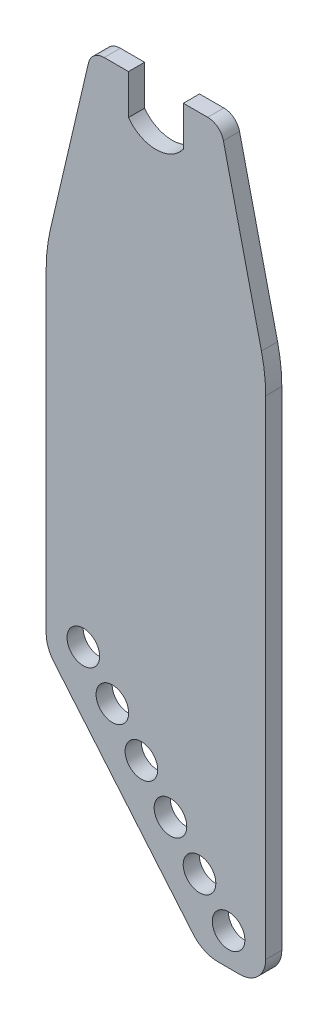
SolidWorks part; units mm, degrees
material "45#"
ref_plane "Front Plane" through (0, 0, 0) normal (0, 0, 1) x (1, 0, 0)
ref_plane "Top Plane" through (0, 0, 0) normal (0, 1, 0) x (1, 0, 0)
ref_plane "Right Plane" through (0, 0, 0) normal (1, 0, 0) x (0, 0, -1)
sketch "Sketch1" plane through (0, 0, 0) normal (0, 0, 1) x (1, 0, 0)
  line L1 (-34, 112.5) -> (34, 112.5)
  line L2 (-34, 112.5) -> (-34, -112.5)
  line L3 (-34, -112.5) -> (34, -112.5)
  line L4 (34, 112.5) -> (34, -112.5)
  line L5 (-34, 112.5) -> (34, -112.5) construction
  line L6 (-34, -112.5) -> (34, 112.5) construction
  point P0 (0, 0)
  dimension "D1" = 68
  dimension "D2" = 225
extrude "Boss-Extrude1" add sketch "Sketch1" along normal blind 5
sketch "Sketch3" plane through (0, 0, 5) normal (0, 0, 1) x (1, 0, 0)
  line L0 (34, -112.5) -> (34, 112.5) construction
  line L1 (-34, -112.5) -> (34, -112.5) construction
  line L2 (22.5, -102.5) -> (-43.0873, -24.336) construction
  circle A0 centre (22.5, -102.5) radius 5.05
  circle A1 centre (13.501, -91.7754) radius 5.05
  circle A2 centre (4.5019, -81.0508) radius 5.05
  circle A3 centre (-4.4971, -70.3261) radius 5.05
  circle A4 centre (-13.4961, -59.6015) radius 5.05
  circle A5 centre (-22.4951, -48.8769) radius 5.05
  dimension "D1" = 10.1
  dimension "D2" = 11.5
  dimension "D3" = 10
  dimension "D5" = 14
  dimension "D9" = 14
  dimension "D4" = 50
  dimension "D6" = 14
  dimension "D7" = 14
  dimension "D8" = 14
extrude "Cut-Extrude1" cut sketch "Sketch3" against normal blind 8
fillet "Fillet1" radius 8 1 edges at (34, -112.5, 2.5)
sketch "Sketch5" plane through (0, 0, 5) normal (0, 0, 1) x (1, 0, 0)
  line L0 (14.5734, -112.5) -> (-34, -54.6125)
  line L1 (-34, -112.5) -> (26, -112.5) construction
  line L2 (-34, -54.6125) -> (-34, -112.5)
  line L3 (-34, -112.5) -> (14.5734, -112.5)
  circle A1 centre (22.5, -102.5) radius 5.05 construction
  dimension "D1" = 50
  dimension "D2" = 12.5
extrude "Cut-Extrude2" cut sketch "Sketch5" against normal through all
fillet "Fillet2" radius 10 1 edges at (14.5734, -112.5, 2.5)
sketch "Sketch6" plane through (0, 0, 5) normal (0, 0, 1) x (1, 0, 0)
  line L1 (-8.5, 112.5) -> (-8.5, 100.1712)
  line L2 (34, 112.5) -> (-34, 112.5) construction
  line L3 (0, 112.5) -> (0, 106.3356) construction
  line L4 (8.5, 112.5) -> (8.5, 100.1712)
  arc A0 (-8.5, 100.1712) -> (8.5, 100.1712) centre (0, 106.3356) ccw
  arc A1 (8.5, 112.5) -> (-8.5, 112.5) centre (0, 106.3356) ccw
  dimension "D1" = 21
  dimension "D2" = 17
extrude "Cut-Extrude3" cut sketch "Sketch6" against normal blind 8
fillet "Fillet3" radius 10 1 edges at (-34, -54.6125, 2.5)
sketch "Sketch7" plane through (0, 0, 5) normal (0, 0, 1) x (1, 0, 0)
  line L0 (-20, 112.5) -> (-34, 52.5)
  line L1 (-8.5, 112.5) -> (-34, 112.5) construction
  line L2 (-34, 112.5) -> (-34, -50.9728) construction
  line L3 (-34, 52.5) -> (-34, 112.5)
  line L4 (-34, 112.5) -> (-20, 112.5)
  line L5 (0, 106.3356) -> (0, 47.5033) construction
  line L6 (34, 112.5) -> (20, 112.5)
  line L7 (34, 52.5) -> (34, 112.5)
  line L8 (20, 112.5) -> (34, 52.5)
  dimension "D1" = 40
  dimension "D2" = 60
extrude "Cut-Extrude4" cut sketch "Sketch7" against normal through all
fillet "Fillet4" radius 5 2 edges at (20, 112.5, 2.5) (-20, 112.5, 2.5)
fillet "Fillet5" radius 50 2 edges at (34, 52.5, 2.5) (-34, 52.5, 2.5)
